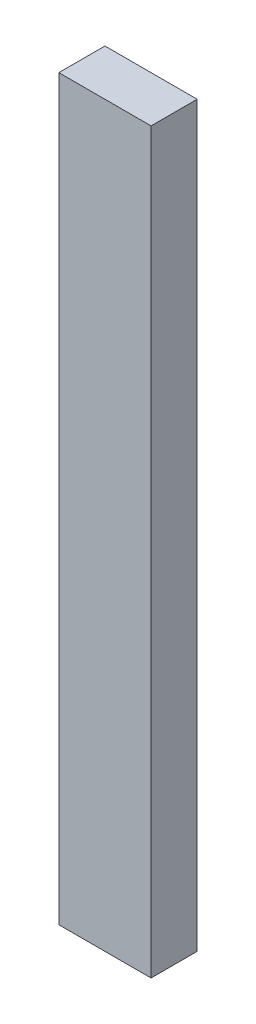
from build123d import *

# Parameters (mm, degrees)
SKETCH1_W          = 10
SKETCH1_H          = 80
BASE_EXTRUDE_DEPTH = 5


with BuildPart() as part:
    # Sketch1 → Base-Extrude (new body)
    with BuildSketch(Plane.XY):
        with Locations((-5, 0)):
            Rectangle(SKETCH1_W, SKETCH1_H)
    extrude(amount=BASE_EXTRUDE_DEPTH)


solid = part.part
